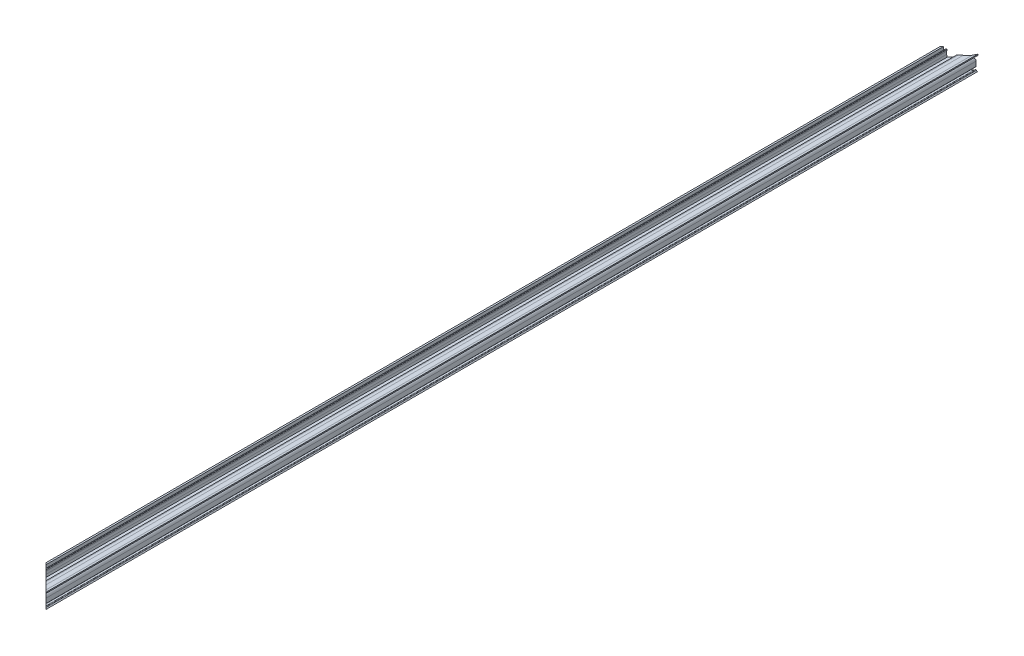
from build123d import *

# Parameters (mm, degrees)
EXTRUDE1_DEPTH      = 1081
EXTRUDE4_DEPTH      = 1083.285410341
EXTRUDE4_DEPTH_BACK = 1083.285410341
EXTRUDE5_DEPTH      = 30


with BuildPart() as part:
    # Sketch2 → Extrude1 (new body)
    with BuildSketch(Plane.XY):
        with BuildLine():
            Line((27.429618111, 61.203514875), (27.429618111, 62.483514875))
            Line((27.429618111, 62.483514875), (27.063725093, 65.097036429))
            ThreePointArc((27.063725093, 65.097036429), (26.9381678, 66.899458408), (27.063725093, 68.701880387))
            Line((27.063725093, 68.701880387), (27.290970266, 70.325060195))
            ThreePointArc((27.290970266, 70.325060195), (27.40740123, 70.522960701), (27.629667144, 70.580568366))
            Line((27.629667144, 70.580568366), (28.223872192, 70.497379659))
            ThreePointArc((28.223872192, 70.497379659), (28.421772697, 70.380948695), (28.479380362, 70.158682782))
            Line((28.479380362, 70.158682782), (28.252135189, 68.535502974))
            ThreePointArc((28.252135189, 68.535502974), (28.1381678, 66.899458408), (28.252135189, 65.263413843))
            Line((28.252135189, 65.263413843), (28.629618111, 62.56710726))
            Line((28.629618111, 62.56710726), (34.119618111, 62.56710726))
            Line((34.119618111, 62.56710726), (34.119618111, 64.76710726))
            Line((34.119618111, 64.76710726), (35.119618111, 64.76710726))
            ThreePointArc((35.119618111, 64.76710726), (36.498022986, 64.671651671), (37.850112572, 64.38710726))
            ThreePointArc((37.850112572, 64.38710726), (40.451975855, 64.047973934), (43.040517634, 64.47710726))
            Line((43.040517634, 64.47710726), (46.429618111, 65.567355231))
            Line((46.429618111, 65.567355231), (46.429618111, 64.306791917))
            Line((46.429618111, 64.306791917), (43.408001834, 63.334760831))
            ThreePointArc((43.408001834, 63.334760831), (40.472780352, 62.848154292), (37.522453236, 63.23270726))
            ThreePointArc((37.522453236, 63.23270726), (36.431587911, 63.468758554), (35.319618111, 63.564834239))
            Line((35.319618111, 63.564834239), (35.319618111, 62.56710726))
            Line((35.319618111, 62.56710726), (41.399618111, 62.56710726))
            ThreePointArc((41.399618111, 62.56710726), (44.228045236, 61.395534384), (45.399618111, 58.56710726))
            Line((45.399618111, 58.56710726), (45.399618111, 53.252873744))
            ThreePointArc((45.399618111, 53.252873744), (45.127835843, 52.807995483), (44.607951444, 52.846757313))
            ThreePointArc((44.607951444, 52.846757313), (41.599927405, 51.269233396), (44.662909839, 49.801265776))
            ThreePointArc((44.662909839, 49.801265776), (45.204517239, 49.836690545), (45.440067721, 49.347702344))
            ThreePointArc((45.440067721, 49.347702344), (45.673249329, 48.549369428), (46.429618111, 48.203514875))
            Line((46.429618111, 48.203514875), (24.429618111, 48.203514875))
            Line((24.429618111, 48.203514875), (24.429618111, 73.203514875))
            Line((24.429618111, 73.203514875), (26.429618111, 73.203514875))
            Line((26.429618111, 73.203514875), (26.429618111, 61.203514875))
            Line((26.429618111, 61.203514875), (27.429618111, 61.203514875))
        make_face()
    extrude(amount=EXTRUDE1_DEPTH)

    # Sketch4 → Extrude4 (cut, two sides: drawn at the far end of the back side and taken through both)
    with BuildSketch(Plane.XZ.offset(-48.203514875).offset(-EXTRUDE4_DEPTH_BACK)):
        Polygon((24.429618111, 0), (46.429618111, 0), (24.429618111, 22), align=None)
    extrude(amount=EXTRUDE4_DEPTH + EXTRUDE4_DEPTH_BACK, mode=Mode.SUBTRACT)

    # Sketch5 → Extrude5 (cut)
    with BuildSketch(Plane.XZ.offset(-48.203514875)):
        Polygon((46.429618111, 1081), (24.429618111, 1059), (24.429618111, 1081), align=None)
    extrude(amount=-EXTRUDE5_DEPTH, mode=Mode.SUBTRACT)


solid = part.part
